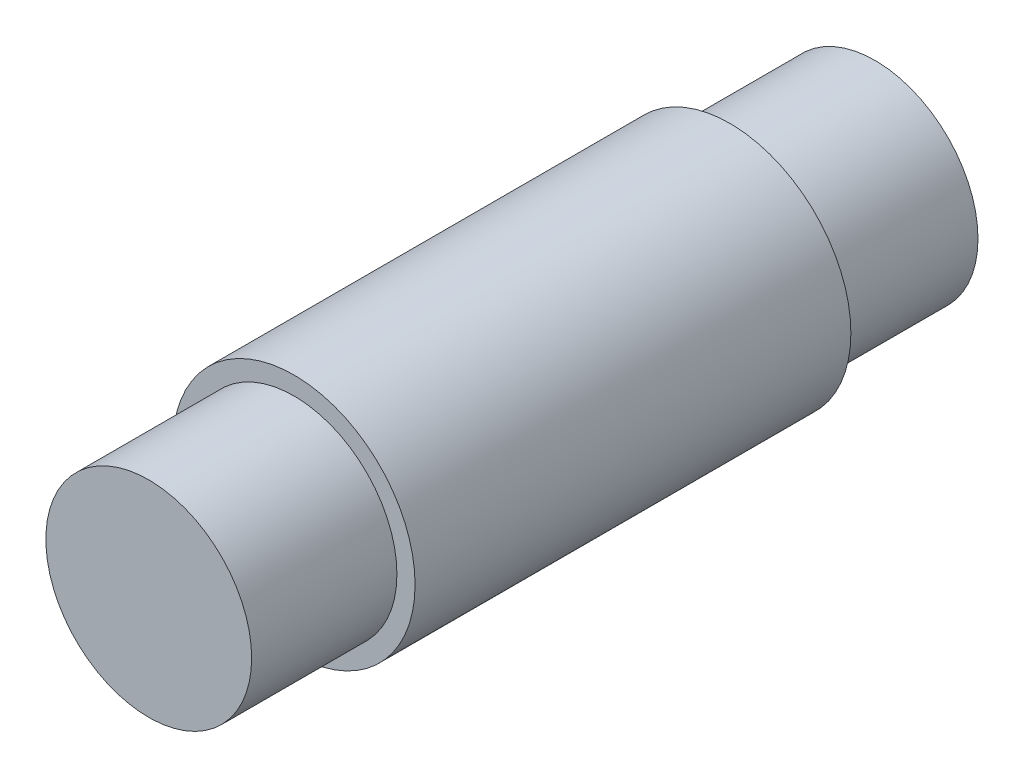
SolidWorks part; units mm, degrees
ref_plane "前视基准面" through (0, 0, 0) normal (0, 0, 1) x (1, 0, 0)
ref_plane "上视基准面" through (0, 0, 0) normal (0, 1, 0) x (1, 0, 0)
ref_plane "右视基准面" through (0, 0, 0) normal (1, 0, 0) x (0, 0, -1)
sketch "草图1" plane through (0, 0, 0) normal (0, 0, 1) x (1, 0, 0)
  circle A0 centre (0, 0) radius 10
  dimension "D1" = 20
extrude "凸台-拉伸1" add sketch "草图1" along normal mid plane 36
sketch "草图2" plane through (0, 0, 18) normal (0, 0, 1) x (1, 0, 0)
  circle A0 centre (0, 0) radius 8.5
  dimension "D1" = 17
extrude "凸台-拉伸2" add sketch "草图2" along normal blind 12
mirror "镜向1" about plane through (0, 0, 0) normal (0, 0, 1) of "凸台-拉伸2"
